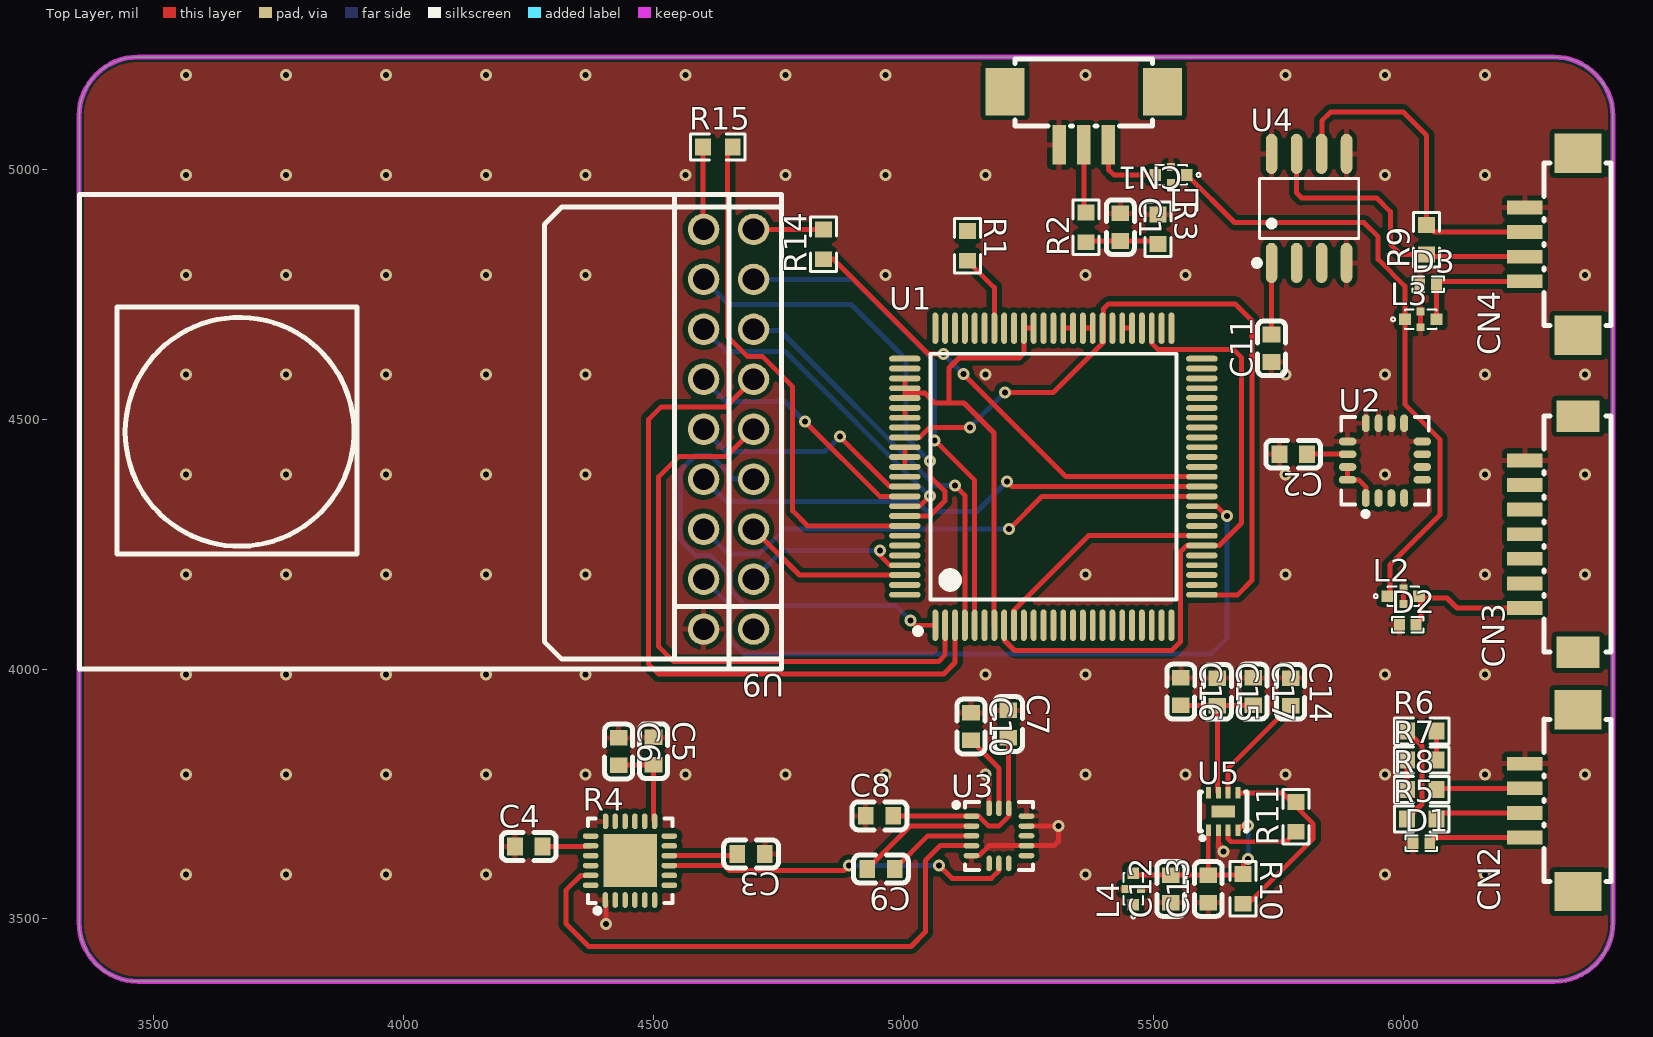
[diagram p0: Top Layer view]
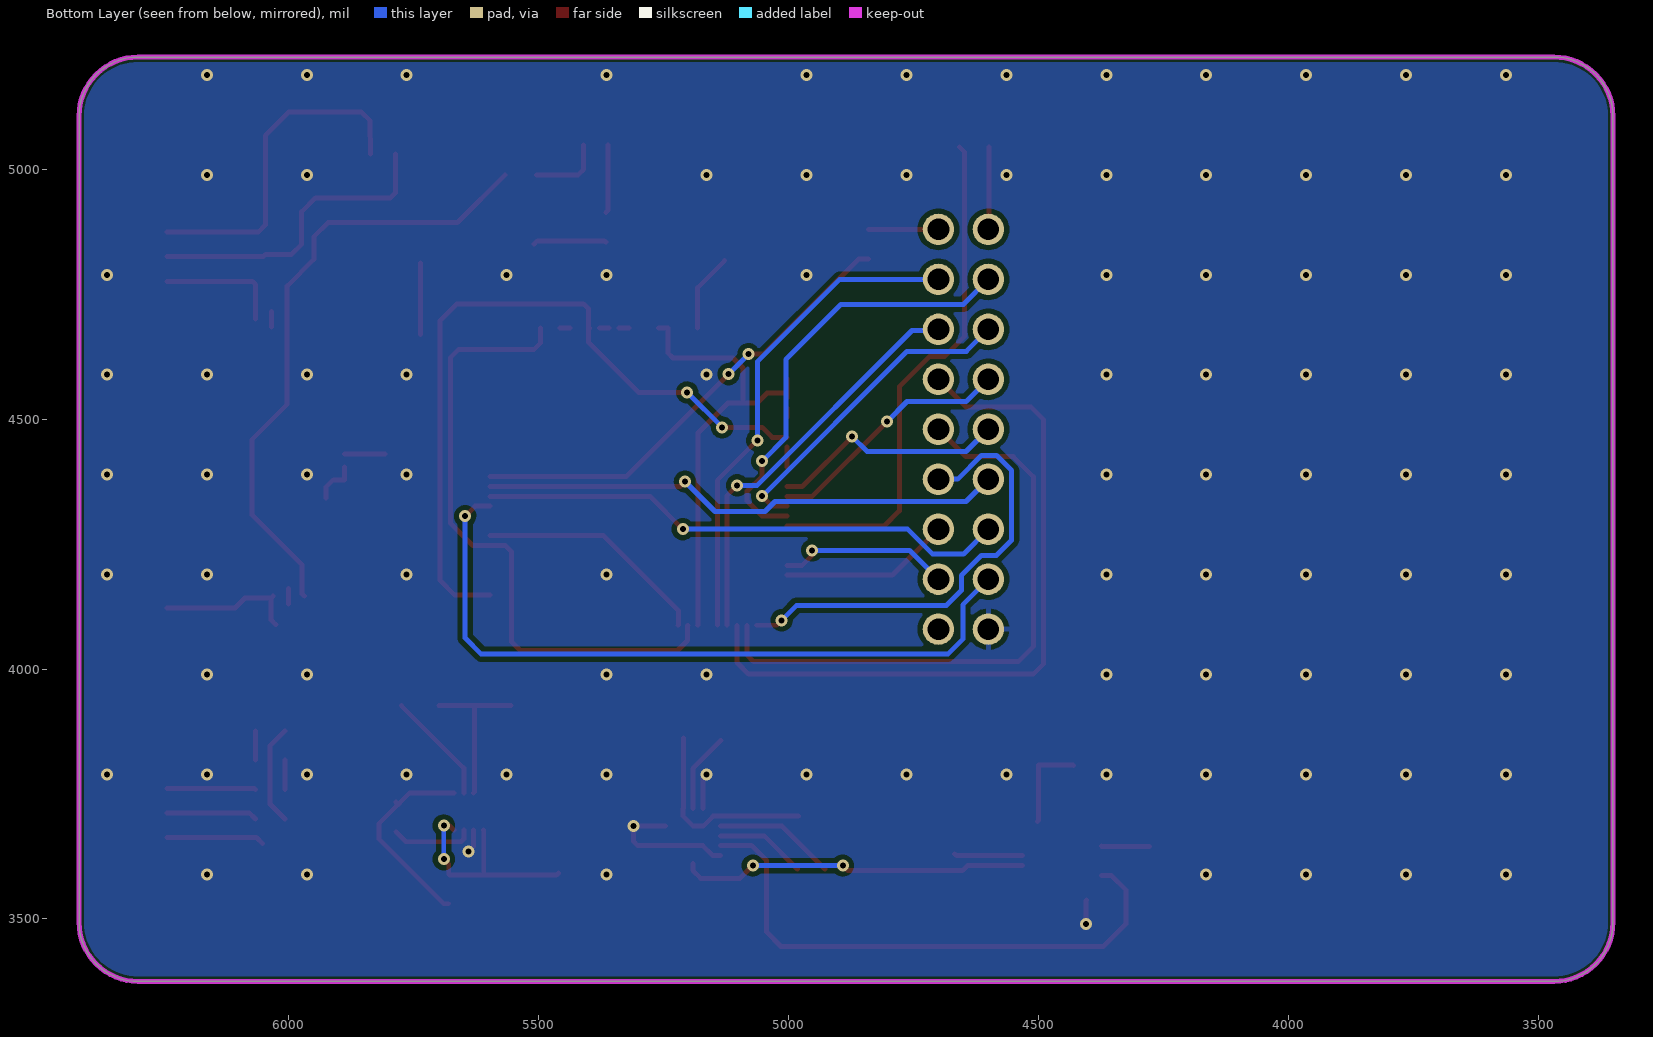
[diagram p1: Bottom Layer view, seen from below]
# Altium PCB MISC50255.pcbdoc
Units mil, origin at the board's own origin, x right, y up, seen from the top; angles counter-clockwise.
Board outline 3070 x 1850 mil, 2 copper layers (Top Layer, Bottom Layer), stack 62.206 mil thick; 47 components, 113 nets, 298 pads, 113 vias.

## Layer stack, top to bottom
Top Solder Mask Layer: solder mask 0.394, Dk 3.3
Top Layer: signal copper 1.379
Dielectric1: surface 59.449, FR4, Dk 4.5
Bottom Layer: signal copper 1.378
Bottom Solder Mask Layer: solder mask 0.394, Dk 3.3

## Board outline
3468.11,5225 ccw(c3468.11,5106.89) 3350,5106.89 3350,3493.11 ccw(c3468.11,3493.11) 3468.11,3375 6301.89,3375 ccw(c6301.89,3493.11) 6420,3493.11 6420,5106.89 ccw(c6301.89,5106.89) 6301.89,5225

## Design rules (kind name [scope] priority, off if disabled: settings)
BoardOutlineClearance copperThickness2oz_1 [All] p2 off: genericclearance=7.99 ignorepadtopadclearanceinfootprint=FALSE except(0: Arc-SplitContinuation Track-SplitContinuation SMDPad-SplitContinuation THPad-SplitContinuation Via-SplitContinuation Fill-SplitContinuation Region-SplitContinuation Poly-SplitContinuation Text-SplitContinuation Hole-SplitContinuation; 5.98: Arc-CutoutEdge Track-CutoutEdge SMDPad-CutoutEdge THPad-CutoutEdge Via-CutoutEdge Text-CutoutEdge; 6.9: Hole-OutlineEdge Hole-CutoutEdge; 10: Poly-OutlineEdge Poly-CutoutEdge; 11.81: Arc-OutlineEdge Track-OutlineEdge SMDPad-OutlineEdge THPad-OutlineEdge Via-OutlineEdge Fill-OutlineEdge Region-OutlineEdge Text-OutlineEdge Fill-CutoutEdge Region-CutoutEdge)
BoardOutlineClearance Plane_innerPlane_1 [All] p4 off: genericclearance=4.02 ignorepadtopadclearanceinfootprint=FALSE except(0: Arc-SplitContinuation Track-SplitContinuation SMDPad-SplitContinuation THPad-SplitContinuation Via-SplitContinuation Fill-SplitContinuation Region-SplitContinuation Poly-SplitContinuation Text-SplitContinuation Hole-SplitContinuation; 5.98: Arc-CutoutEdge Track-CutoutEdge SMDPad-CutoutEdge THPad-CutoutEdge Via-CutoutEdge Text-CutoutEdge; 6.9: Hole-OutlineEdge Hole-CutoutEdge; 10: Poly-OutlineEdge Poly-CutoutEdge; 11.81: Arc-OutlineEdge Track-OutlineEdge SMDPad-OutlineEdge THPad-OutlineEdge Via-OutlineEdge Fill-OutlineEdge Region-OutlineEdge Text-OutlineEdge Fill-CutoutEdge Region-CutoutEdge)
BoardOutlineClearance Copper_copperRegion_1 [All] p6 off: genericclearance=4.02 ignorepadtopadclearanceinfootprint=FALSE except(0: Arc-SplitContinuation Track-SplitContinuation SMDPad-SplitContinuation THPad-SplitContinuation Via-SplitContinuation Fill-SplitContinuation Region-SplitContinuation Poly-SplitContinuation Text-SplitContinuation Hole-SplitContinuation; 5.98: Arc-CutoutEdge Track-CutoutEdge SMDPad-CutoutEdge THPad-CutoutEdge Via-CutoutEdge Text-CutoutEdge; 6.9: Hole-OutlineEdge Hole-CutoutEdge; 10: Poly-OutlineEdge Poly-CutoutEdge; 11.81: Arc-OutlineEdge Track-OutlineEdge SMDPad-OutlineEdge THPad-OutlineEdge Via-OutlineEdge Fill-OutlineEdge Region-OutlineEdge Text-OutlineEdge Fill-CutoutEdge Region-CutoutEdge)
BoardOutlineClearance copperThickness1oz_1 [All] p8: genericclearance=4.02 ignorepadtopadclearanceinfootprint=FALSE except(0: Arc-SplitContinuation Track-SplitContinuation SMDPad-SplitContinuation THPad-SplitContinuation Via-SplitContinuation Fill-SplitContinuation Region-SplitContinuation Poly-SplitContinuation Text-SplitContinuation Hole-SplitContinuation; 5.98: Arc-CutoutEdge Track-CutoutEdge SMDPad-CutoutEdge THPad-CutoutEdge Via-CutoutEdge Text-CutoutEdge; 6.9: Hole-OutlineEdge Hole-CutoutEdge; 10: Poly-OutlineEdge Poly-CutoutEdge; 11.81: Arc-OutlineEdge Track-OutlineEdge SMDPad-OutlineEdge THPad-OutlineEdge Via-OutlineEdge Fill-OutlineEdge Region-OutlineEdge Text-OutlineEdge Fill-CutoutEdge Region-CutoutEdge)
Clearance copperThickness2oz [All] p1 off: gap=7.99 ignorepadtopadclearanceinfootprint=FALSE except(5.98: SMDPad-Track SMDPad-SMDPad THPad-Track SMDPad-THPad THPad-THPad Track-Via SMDPad-Via THPad-Via Via-Via Fill-SMDPad Region-SMDPad Fill-THPad Region-THPad Fill-Via Region-Via Fill-Fill Fill-Region Region-Region Arc-Track Arc-SMDPad Arc-THPad Arc-Via Fill-Arc Region-Arc Arc-Arc Text-Track SMDPad-Text Text-THPad Text-Via Fill-Text Region-Text Arc-Text Text-Text; 6.9: Hole-Track Hole-SMDPad Hole-THPad Hole-Via Fill-Hole Region-Hole Hole-Arc Hole-Text; 10: Poly-Track Poly-SMDPad Poly-THPad Poly-Via Poly-Fill Poly-Region Poly-Poly Poly-Arc Poly-Text Poly-Hole; 11.81: Fill-Track Region-Track)
Clearance Plane_innerPlane [All] p3 off: gap=4.02 ignorepadtopadclearanceinfootprint=FALSE except(5.98: SMDPad-Track SMDPad-SMDPad THPad-Track SMDPad-THPad THPad-THPad Track-Via SMDPad-Via THPad-Via Via-Via Fill-SMDPad Region-SMDPad Fill-THPad Region-THPad Fill-Via Region-Via Fill-Fill Fill-Region Region-Region Arc-Track Arc-SMDPad Arc-THPad Arc-Via Fill-Arc Region-Arc Arc-Arc Text-Track SMDPad-Text Text-THPad Text-Via Fill-Text Region-Text Arc-Text Text-Text; 6.9: Hole-Track Hole-SMDPad Hole-THPad Hole-Via Fill-Hole Region-Hole Hole-Arc Hole-Text; 10: Poly-Track Poly-SMDPad Poly-THPad Poly-Via Poly-Fill Poly-Region Poly-Poly Poly-Arc Poly-Text Poly-Hole; 11.81: Fill-Track Region-Track)
Clearance Copper_copperRegion [All] p5 off: gap=4.02 ignorepadtopadclearanceinfootprint=FALSE except(5.98: SMDPad-Track SMDPad-SMDPad THPad-Track SMDPad-THPad THPad-THPad Track-Via SMDPad-Via THPad-Via Via-Via Fill-SMDPad Region-SMDPad Fill-THPad Region-THPad Fill-Via Region-Via Fill-Fill Fill-Region Region-Region Arc-Track Arc-SMDPad Arc-THPad Arc-Via Fill-Arc Region-Arc Arc-Arc Text-Track SMDPad-Text Text-THPad Text-Via Fill-Text Region-Text Arc-Text Text-Text; 6.9: Hole-Track Hole-SMDPad Hole-THPad Hole-Via Fill-Hole Region-Hole Hole-Arc Hole-Text; 10: Poly-Track Poly-SMDPad Poly-THPad Poly-Via Poly-Fill Poly-Region Poly-Poly Poly-Arc Poly-Text Poly-Hole; 11.81: Fill-Track Region-Track)
Clearance copperThickness1oz [All] p7: gap=4.02 ignorepadtopadclearanceinfootprint=FALSE except(5.98: SMDPad-Track SMDPad-SMDPad THPad-Track SMDPad-THPad THPad-THPad Track-Via SMDPad-Via THPad-Via Via-Via Fill-SMDPad Region-SMDPad Fill-THPad Region-THPad Fill-Via Region-Via Fill-Fill Fill-Region Region-Region Arc-Track Arc-SMDPad Arc-THPad Arc-Via Fill-Arc Region-Arc Arc-Arc Text-Track SMDPad-Text Text-THPad Text-Via Fill-Text Region-Text Arc-Text Text-Text; 6.9: Hole-Track Hole-SMDPad Hole-THPad Hole-Via Fill-Hole Region-Hole Hole-Arc Hole-Text; 10: Poly-Track Poly-SMDPad Poly-THPad Poly-Via Poly-Fill Poly-Region Poly-Poly Poly-Arc Poly-Text Poly-Hole; 11.81: Fill-Track Region-Track)
DiffPairsRouting differentialPair [All] p1: maxlimit=6 minlimit=6 mostfreqgap=6 toplayer_minwidth=5 toplayer_prefwidth=10 toplayer_maxwidth=100 toplayer_mingap=6 toplayer_prefgap=6 toplayer_maxgap=6 bottomlayer_minwidth=5 bottomlayer_prefwidth=10 bottomlayer_maxwidth=100 bottomlayer_mingap=6 bottomlayer_prefgap=6 bottomlayer_maxgap=6 maxuncoupledlength=10
HoleToHoleClearance otherClearance [All] p1: gap=11.81 allowstackedmicrovias=TRUE
Length netLength [All] p1: minlimit=0 maxlimit=0
PasteMaskExpansion pasteMaskExpansion [All] p1: expansion=0
PlaneConnect innerPlane [All] p1: planeconnectstyle=Relief reliefexpansion=20 reliefentries=4 reliefconductorwidth=10 reliefairgap=10
PolygonConnect copperRegion [All] p1: connectstyle=Relief reliefconductorwidth=10 reliefentries=4 polygonreliefangle="90 Angle" airgapwidth=10 via.connectstyle=Relief via.reliefconductorwidth=10 via.reliefentries=4 via.polygonreliefangle="90 Angle" via.airgapwidth=10
RoutingVias viaSize [All] p1: holewidth=12.01 width=24.02 viastyle="Through Hole" minholewidth=11.81 minwidth=19.68 maxholewidth=248.03 maxwidth=393.7
SolderMaskExpansion solderMaskExpansion [IsVia] p1: expansion=-1000 istentingtop=TRUE
SolderMaskExpansion solderMaskExpansion [All] p2: expansion=2 istentingtop=FALSE
Width copperThickness2oz_2 [All] p1 off: maxlimit=100 minlimit=8 preferedwidth=10
Width copperThickness1oz_2 [All] p2: maxlimit=100 minlimit=5 preferedwidth=10

## Components (designator, comment, footprint, x,y, rotation, side; value= is the part's Value field where it differs from the comment)
C1 "100nF" C0603 5433.99,4884.53 r270 top
C2 "10nF" C0603 5780,4430 r180 top
C3 "2U2" C0603 4695,3630 r180 top
C4 "2U2" C0603 4250,3645 r0 top
C5 "2U2" C0603 4499.92,3835.89 r270 top
C6 "0U1" C0603 4430,3835 r270 top
C7 "10UF" C0603 5210,3890 r270 top
C8 "10UF" C0603 4952.03,3706.27 r0 top
C9 "10UF" C0603 4955,3600 r180 top
C10 "10UF" C0603 5135,3885 r270 top
C11 "100nF" C0603 5736.72,4642.03 r90 top
C12 "100nF" C0603 5535,3560 r90 top
C13 "100nF" C0603 5610,3560 r90 top
C14 "100nF" C0603 5774.86,3954.38 r270 top
C15 "100nF" C0603 5628.17,3954.38 r270 top
C16 "100nF" C0603 5555,3955 r270 top
C17 "100nF" C0603 5700,3955 r270 top
CN1 "DF13C-3P-1.25V(51)" CONN-SMD_3P-P1.25_DF13C-3P-1.25V 5360.82,5102.4 r180 top
CN2 "DF13C-4P-1.25V(51)" CONN-SMD_4P-P1.25_DF13C-4P-1.25V 6296.86,3736.86 r90 top
CN3 "DF13C-7P-1.25V(51)" CONN-SMD_7P-P1.25_DF13C-7P-1.25V 6296.86,4270 r90 top
CN4 "DF13C-4P-1.25V(51)" CONN-SMD_4P-P1.25_DF13C-4P-1.25V 6296.86,4850 r90 top
D1 "PESD0402-05ST-ES" DFN1006-2L-BI 6036.51,3651.42 r0 top
D2 "PESD0402-05ST-ES" DFN1006-2L-BI 6009.24,4088.91 r0 top
D3 "PESD0402-05ST-ES" DFN1006-2L-BI 6050,4770 r0 top
L1 "KNH16C104DA5TS" FILTER-SMD_3P-L1.6-W0.8_YFF18PCXXXXXXX 5535.53,4989.03 r180 top
L2 "KNH16C104DA5TS" FILTER-SMD_3P-L1.6-W0.8_YFF18PCXXXXXXX 6000.37,4145.95 r0 top
L3 "KNH16C104DA5TS" FILTER-SMD_3P-L1.6-W0.8_YFF18PCXXXXXXX 6035,4700 r0 top
L4 "KNH16C104DA5TS" FILTER-SMD_3P-L1.6-W0.8_YFF18PCXXXXXXX 5460,3560 r90 top
R1 "10K" R0603 5127.87,4847.02 r270 top
R2 "10K" R0603 5365.53,4884.03 r90 top
R3 "10K" R0603 5508.97,4880.31 r270 top
R4 "MPU-6000" QFN-24_L4.0-W4.0-P0.50-BL-EP2.7 4452.65,3616.63 r0 top
R5 "120R" R0603 6037.28,3700 r0 top
R6 "120R" R0603 6037.28,3876.42 r0 top
R7 "120R" R0603 6037.28,3817.61 r0 top
R8 "120R" R0603 6037.28,3758.81 r0 top
R9 "120R" R0603 6046.83,4859.48 r90 top
R10 "120R" R0603 5680,3560 r270 top
R11 "10K" R0603 5785.47,3704.08 r90 top
R14 "10K" R0603 4840,4850 r90 top
R15 "10K" R0603 4628.56,5045.17 r0 top
U1 "STM32F427VGT6" LQFP-100_L14.0-W14.0-P0.50-LS16.0-BL 5300,4385 r0 top
U2 "L3GD20" LGA-16_L4.0-W4.0-P0.65-BL 5963.7,4417.23 r0 top
U3 "LSM303D" LGA-16_L3.0-W3.0-P0.50-TL 5191.1,3666.27 r0 top
U4 "MAX3051ESA+T" SOIC-8_L4.9-W3.9-P1.27-LS6.0-BL 5811.72,4922.03 r0 top
U5 "MIC5332-PPYMT-TR" MLF-8_L2.0-W2.0-P0.50-BL-EP 5640,3715 r0 top
U9 "OV2640 Camera Board" SENSORM-TH_L35.7-W3.9-OV2640 4650,4480 r180 top

## Footprints (in the part's own frame and the unit in brackets; to place one, negate y for a bottom-side part, rotate by r counter-clockwise, add the part's x,y. Pads: shape width x height; smd on the part's side, far side on the other; paste and mask are expansions set on the pad)
C0603 [mm]
  rect 0.8x0.9 smd: 1(-0.7,0) 2(0.7,0)
  silkscreen extent -1.39,-0.71 1.39,0.71
CONN-SMD_3P-P1.25_DF13C-3P-1.25V [mm]
  rect 0.7x2 smd: 1(-1.25,1.35) 2(0,1.35) 3(1.25,1.35)
  rect 2x2.4 smd: 4(4,-1.35) 5(-4,-1.35)
  silkscreen extent -3.5,-3.02 3.5,0.38
CONN-SMD_4P-P1.25_DF13C-4P-1.25V [mm]
  rect 0.7x1.8 smd: 1(-1.875,1.35) 2(-0.625,1.35) 3(0.625,1.35) 4(1.875,1.35)
  rect 2x2.4 smd: 5(4.625,-1.35) 6(-4.625,-1.35)
  silkscreen extent -4.13,-3.02 4.14,0.38
CONN-SMD_7P-P1.25_DF13C-7P-1.25V [mm]
  rect 0.7x1.8 smd paste+0 mask+0.05: 1(-3.75,1.35) 2(-2.5,1.35) 3(-1.25,1.35) 4(0,1.35) 5(1.25,1.35) 6(2.5,1.35) 7(3.75,1.35)
  rect 1.6x2.2 smd paste+0 mask+0.05: 8(6,-1.35) 9(-6,-1.35)
  silkscreen extent -6,-3.02 6,0.38
DFN1006-2L-BI [mm]
  rect 0.55x0.6 smd: 1(-0.425,0) 2(0.425,0)
  silkscreen extent -0.8,-0.4 0.8,0.4
FILTER-SMD_3P-L1.6-W0.8_YFF18PCXXXXXXX [mm]
  rect 0.6x0.6 smd: 1(-0.8,0) 3(0.8,0)
  rect 0.4x0.4 smd: 2(0,0.4) 2(0,-0.4)
  silkscreen extent -1.5,-0.5 0.8,0.5
LGA-16_L3.0-W3.0-P0.50-TL [mm]
  oval 0.8x0.28 smd: 1(-1.4,1) 2(-1.4,0.5) 3(-1.4,0) 4(-1.4,-0.5) 5(-1.4,-1) 9(1.4,-1) 10(1.4,-0.5) 11(1.4,0) 12(1.4,0.5) 13(1.4,1)
  oval 0.28x0.8 smd: 6(-0.5,-1.4) 7(0,-1.4) 8(0.5,-1.4) 14(0.5,1.4) 15(0,1.4) 16(-0.5,1.4)
  silkscreen extent -2.3,-1.72 1.73,1.73
LGA-16_L4.0-W4.0-P0.65-BL [mm]
  oval 0.4x0.9 smd: 1(-0.975,-1.9) 2(-0.325,-1.9) 3(0.325,-1.9) 4(0.975,-1.9) 9(0.975,1.9) 10(0.325,1.9) 11(-0.325,1.9) 12(-0.975,1.9)
  oval 0.9x0.4 smd: 5(1.9,-0.975) 6(1.9,-0.325) 7(1.9,0.325) 8(1.9,0.975) 13(-1.9,0.975) 14(-1.9,0.325) 15(-1.9,-0.325) 16(-1.9,-0.975)
  silkscreen extent -2.22,-2.84 2.22,2.22
LQFP-100_L14.0-W14.0-P0.50-LS16.0-BL [mm]
  oval 0.3x1.6 smd: 1(-6,-7.55) 2(-5.5,-7.55) 3(-5,-7.55) 4(-4.5,-7.55) 5(-4,-7.55) 6(-3.5,-7.55) 7(-3,-7.55) 8(-2.5,-7.55) 9(-2,-7.55) 10(-1.5,-7.55) 11(-1,-7.55) 12(-0.5,-7.55) 13(0,-7.55) 14(0.5,-7.55) 15(1,-7.55) 16(1.5,-7.55) 17(2,-7.55) 18(2.5,-7.55) 19(3,-7.55) 20(3.5,-7.55) 21(4,-7.55) 22(4.5,-7.55) 23(5,-7.55) 24(5.5,-7.55) 25(6,-7.55) 51(6,7.55) 52(5.5,7.55) 53(5,7.55) 54(4.5,7.55) 55(4,7.55) 56(3.5,7.55) 57(3,7.55) 58(2.5,7.55) 59(2,7.55) 60(1.5,7.55) 61(1,7.55) 62(0.5,7.55) 63(0,7.55) 64(-0.5,7.55) 65(-1,7.55) 66(-1.5,7.55) 67(-2,7.55) 68(-2.5,7.55) 69(-3,7.55) 70(-3.5,7.55) 71(-4,7.55) 72(-4.5,7.55) 73(-5,7.55) 74(-5.5,7.55) 75(-6,7.55)
  oval 1.6x0.3 smd: 26(7.55,-6) 27(7.55,-5.5) 28(7.55,-5) 29(7.55,-4.5) 30(7.55,-4) 31(7.55,-3.5) 32(7.55,-3) 33(7.55,-2.5) 34(7.55,-2) 35(7.55,-1.5) 36(7.55,-1) 37(7.55,-0.5) 38(7.55,0) 39(7.55,0.5) 40(7.55,1) 41(7.55,1.5) 42(7.55,2) 43(7.55,2.5) 44(7.55,3) 45(7.55,3.5) 46(7.55,4) 47(7.55,4.5) 48(7.55,5) 49(7.55,5.5) 50(7.55,6) 76(-7.55,6) 77(-7.55,5.5) 78(-7.55,5) 79(-7.55,4.5) 80(-7.55,4) 81(-7.55,3.5) 82(-7.55,3) 83(-7.55,2.5) 84(-7.55,2) 85(-7.55,1.5) 86(-7.55,1) 87(-7.55,0.5) 88(-7.55,0) 89(-7.55,-0.5) 90(-7.55,-1) 91(-7.55,-1.5) 92(-7.55,-2) 93(-7.55,-2.5) 94(-7.55,-3) 95(-7.55,-3.5) 96(-7.55,-4) 97(-7.55,-4.5) 98(-7.55,-5) 99(-7.55,-5.5) 100(-7.55,-6)
  silkscreen extent -7.03,-8 6.25,6.25
MLF-8_L2.0-W2.0-P0.50-BL-EP [mm]
  rect 0.25x0.6 smd: 1(-0.75,-0.95) 2(-0.25,-0.95) 3(0.25,-0.95) 4(0.75,-0.95) 5(0.75,0.95) 6(0.25,0.95) 7(-0.25,0.95) 8(-0.75,0.95)
  rect 1.2x0.6 smd: 9(0,0)
  silkscreen extent -1.2,-1.45 1.2,1
QFN-24_L4.0-W4.0-P0.50-BL-EP2.7 [mm]
  oval 0.28x0.8 smd paste-100 mask+0.05: 1(-1.25,-2) 2(-0.75,-2) 3(-0.25,-2) 4(0.25,-2) 5(0.75,-2) 6(1.25,-2) 13(1.25,2) 14(0.75,2) 15(0.25,2) 16(-0.25,2) 17(-0.75,2) 18(-1.242,2)
  oval 0.8x0.28 smd paste-100 mask+0.05: 7(2,-1.25) 8(2,-0.75) 9(2,-0.25) 10(2,0.25) 11(2,0.75) 12(2,1.25) 19(-2,1.25) 20(-2,0.75) 21(-2,0.25) 22(-2,-0.25) 23(-2,-0.75) 24(-2,-1.25)
  rect 2.7x2.7 smd paste-100 mask+0.05: 25(0.012,0)
  silkscreen extent -2.14,-2.79 2.16,2.15
R0603 [mil]
  rect 31.75x34.02 smd paste-3937.01 mask+2: 1(-29.66,0) 2(29.66,0)
  silkscreen extent -55,-26 55,26
SENSORM-TH_L35.7-W3.9-OV2640 [mm]
  round 1.6 hole 1.1 paste+0 mask+0.05: 1(-1.27,10.16) 2(-1.27,7.62) 3(-1.27,5.08) 4(-1.27,2.54) 5(-1.27,0) 6(-1.27,-2.54) 7(-1.27,-5.08) 8(-1.27,-7.62) 9(-1.27,-10.16) 10(1.27,-10.16) 11(1.27,-7.62) 12(1.27,-5.08) 13(1.27,-2.54) 14(1.27,0) 15(1.27,2.54) 16(1.27,5.08) 17(1.27,7.62) 18(1.27,10.16)
  silkscreen extent -2.7,-11.94 32.99,12.19
SOIC-8_L4.9-W3.9-P1.27-LS6.0-BL [mm]
  oval 0.588x2.045 smd: 1(-1.905,-2.772) 2(-0.635,-2.772) 3(0.635,-2.772) 4(1.905,-2.772) 5(1.905,2.772) 6(0.635,2.772) 7(-0.635,2.772) 8(-1.905,2.772)
  silkscreen extent -2.8,-2.92 2.53,1.52

## Via types
v1: diameter 24.02, hole 12, Top Layer to Bottom Layer, 113 vias

## Nets (pads, with @x,y where several pads share a name; then routed paths per layer and width w, separated by ;. In a path a pad name is that pad's centre, name@x,y a point inside that pad or via, vN(x,y) a via of type N, cw(c..) or ccw(c..) an arc to the next point about the centre after c; other vN are vias at no path point)
$1N877: R1.2 U1.69 | length 157.5
  Top Layer w10: R1.2 5181.89,4763.34 U1.69
$1N1241: CN1.1 L1.3 | length 147.8
  Top Layer w10: CN1.1 5410.03,4999.97 5420.97,4989.03 L1.3
$1N1807: C2.1 U2.14 | length 81.3
  Top Layer w10: C2.1 U2.14
$1N2279: C3.2 R4.10 | length 137.5
  Top Layer w10: R4.10 4663.91,3626.47 C3.2
$1N2414: C4.2 R4.20 | length 96.8
  Top Layer w10: C4.2 4372.75,3645 R4.20
$1N3306: C9.1 U3.3 | length 180.9
  Top Layer w10: C9.1 5048.84,3666.28 U3.3
$1N3316: C9.2 U3.2 | length 244.1
  Top Layer w10: C9.2 5013.4,3685.96 U3.2
$1N3418: C10.2 U3.15 | length 159.3
  Top Layer w10: C10.2 5191.1,3801.34 U3.15
$1N3634: CN2.1 D1.2 | length 195.3
  Top Layer w10: D1.2 6064.85,3663.04 CN2.1
$1N3639: CN2.2 R5.2 | length 181.8
  Top Layer w10: R5.2 6079.19,3712.25 CN2.2
$1N3808: CN2.3 R8.2 | length 177.9
  Top Layer w10: R8.2 6069.59,3761.46 CN2.3
$1N4095: CN3.1 D2.2 L2.3 | length 279
  Top Layer w10: D2.2 6035.47,4098.4 L2.3@6035.47,4142.36 ; L2.3 L2.3@6035.47,4142.36 ; CN3.1 6107.64,4122.36 6087.64,4142.36 L2.3@6035.47,4142.36
$1N4583: CN4.1 D3.2 L3.3 | length 249.3
  Top Layer w10: L3.3@6066.73,4700.23 D3.2 6072.9,4776.18 CN4.1
$1N6097: C12.2 C13.2 L4.3 R10.1 U5.1 U5.4 | length 438.8
  Top Layer w9.84: C13.2 5610,3677.13 U5.1 ; U5.4 5679.06,3687.13 v1(5690,3687.13) ; R10.1 5680,3609.66 v1(5690,3619.66)
  Top Layer w10: L4.3 5463.94,3587.56 C12.2 C13.2 5677.9,3587.56 R10.1
  Bottom Layer w9.84: v1(5690,3619.66) v1(5690,3687.13)
$1N6348: C14.2 U5.6 | length 226.2
  Top Layer w9.84: U5.6 5649.84,3801.8 C14.2
$1N10490: R14.2 U9.9 | length 140.1
  Top Layer w10: U9.9 4700.34,4879.66 R14.2
$1N10540: R15.1 U9.10 | length 165.6
  Top Layer w10: R15.1 4598.9,4881.1 U9.10
(RPUCS/5.1C: U1.17
ACCELDRDY/1.1B: U3.11
ACCELHAGCS/1.3B: U3.8
ALARM/7.10: U1.77
BAROCS/5.40: U1.88
BATT_CURRENT_SENS//11.2C: U1.26 U1.58 U1.84 | length 1492.4
  Top Layer w10: U1.84 5032.76,4463.74 5052.76,4483.74 v1(5132.76,4483.74) ; v1(5202.76,4553.74) 5299.93,4553.74 5399.93,4653.74 U1.58@5399.93,4680.74 ; U1.58 U1.58@5399.93,4680.74 ; U1.26 5668.78,4148.78 5697.24,4177.24 5697.24,4697.76 5664.26,4730.74 5409.93,4730.74 5399.93,4720.74 U1.58@5399.93,4680.74
  Bottom Layer w10: v1(5132.76,4483.74) v1(5202.76,4553.74)
BATT_VOLTAGE_SENS/11.2C: U1.25
CAN1-X/4.4C: U1.81 U1.82 | length 19.7
  Top Layer w10: U1.82 U1.81
CAN1_RX/1.3B: U4.3
CAN1TX/1.3B: U4.2
CAN2RX/2.4C: U1.51
CANH/12.3C: CN4.2 R9.1 U4.7 | length 625.9
  Top Layer w10: U4.7 5786.72,4953.28 5796.72,4943.28 5946.72,4943.28 5974.43,4915.57 5974.43,4850.57 5995.18,4829.82 R9.1 6051.27,4825.39 CN4.2
CANL/12.3C: CN4.3 R9.2 U4.6 | length 684.4
  Top Layer w10: U4.6 5837.14,5097.14 5855,5115 6000,5115 6046.83,5068.17 R9.2 6061.38,4874.6 CN4.3
CBUSUALID/11.6C: U1.15
CU003U3SENS0RS/12.6A: U5.8
D2: U1.92 U9.11 | length 879.6
  Top Layer w10: U1.92 5052.76,4306.26 5082.76,4336.26 5082.76,4356.26 5052.76,4386.26 v1(5052.76,4416.26)
  Bottom Layer w10: U9.11 4650,4730 4895,4730 5005,4620 5005,4464.02 v1(5052.76,4416.26)
D3: U1.5 U9.8 | length 991.4
  Top Layer w10: v1(5062.52,4457.76) 5142.52,4377.76 U1.5
  Bottom Layer w10: U9.8 4897.82,4780 5062.52,4615.3 v1(5062.52,4457.76)
D4: U1.91 U9.12 | length 649.4
  Top Layer w10: U1.91 5032.76,4325.94 v1(5052.76,4345.94)
  Bottom Layer w10: U9.12 4644.06,4635.94 4762.76,4635.94 v1(5052.76,4345.94)
D5: U1.4 U9.7 | length 820.4
  Top Layer w10: v1(5102.83,4367.76) 5122.83,4347.76 U1.4
  Bottom Layer w10: U9.7 4702.24,4677.76 4752.83,4677.76 5062.83,4367.76 v1(5102.83,4367.76)
D6: U1.90 U9.13 | length 499.8
  Top Layer w10: v1(4802.76,4495.63) 4952.76,4345.63 U1.90
  Bottom Layer w10: U9.13 4644.37,4535.63 4762.76,4535.63 v1(4802.76,4495.63)
D7: U1.3 U9.6 | length 1438.8
  Top Layer w10: U9.6 4645,4525 4515,4525 4490,4500 4490,4010 4510,3990 5080,3990 5103.15,4013.15 U1.3
D8: U1.89 U9.14 | length 475.1
  Top Layer w10: v1(4872.76,4465.32) 4972.76,4365.32 U1.89
  Bottom Layer w10: U9.14 4644.68,4435.32 4842.76,4435.32 v1(4872.76,4465.32)
D9: U1.2 U9.5 | length 1220.1
  Top Layer w10: U9.5 4645,4425 4550,4425 4510,4385 4510,4045 4540,4015 5070,4015 5083.46,4028.46 U1.2
FHU-5MCLK/3.5C: U1.76
FHU-12C1SOAV4.10: U1.96
FHU-CHSV9.1A: U1.61 U1.62 | length 19.7
  Top Layer w10: U1.62 U1.61
FHU-RLSET/7.1B: R11.1 U5.3 | length 163.8
  Top Layer w9.84: U5.3 5649.84,3660.05 5655.47,3654.42 5765.47,3654.42 R11.1
FHU-UDD3U3/7.38: C15.2 C16.2 C17.2 U5.7 | length 320.8
  Top Layer w9.84: C15.2 5628.17,3754.39 U5.7
  Top Layer w10: C16.2 5555.62,3926.82 C15.2 5699.38,3926.82 C17.2
FHU-USART2CTS/2.18: U1.85 U1.86 U1.87 | length 39.4
  Top Layer w10: U1.87 U1.86 U1.85
FHU-USART3_CTS/2.1A: U1.59 U1.60 | length 19.7
  Top Layer w10: U1.60 U1.59
FHU-USART3TX/2.1A: U1.55 U1.56 | length 19.7
  Top Layer w10: U1.56 U1.55
FHUAUKADC1/4.48: U1.18
FHUAUKADC2/4.4A: U1.33
FMU-12C1SCL/4.10: U1.95
FMU-12C2_SCL/3.4A: U1.47
FMU-12C2_SDA/3.4A: U1.48
FMU-I2C1_SCL/1.1C: R5.1 R6.1 | length 201.3
  Top Layer w10: R5.1 6037.62,3730 6037.62,3846.42 R6.1
FMU-I2C1_SDA/1.1C: R7.1 R8.1 | length 58.8
  Top Layer w10: R8.1 R7.1
FMU-SHD10/3.5C: U1.72
FMU-UART4_RX/2.1C: U1.24
FMU-UART4_TX/2.1C: U1.23
FMU-UDD_3U3/3.5C: C11.2 U4.1 | length 143.3
  Top Layer w10: C11.2 U4.1
FMU-VDD_3U3/3.50: R6.2 R7.2 | length 58.8
  Top Layer w10: R7.2 R6.2
FRAMCS: U1.57
FRAMMOSI: U1.54
FRAMSCK: U1.52
GND: C1.1 C2.2 C3.1 C4.1 C5.1 C6.1 C7.1 C8.1 C10.1 C11.1 C12.1 C13.1 C14.1 C15.1 C16.1 C17.1 CN1.3 CN2.4 CN3.7 CN4.4 D1.1 D2.1 D3.1 L1.2 L2.2 L3.2 L4.2 R3.1 R4.1 R4.18 U2.8 U2.9 U2.10 U2.11 U2.12 U2.13 U3.5 U3.10 U3.12 U3.13 U3.16 U4.4 U4.5 U4.8 U5.2 U9.18 | length 509.4
  Top Layer w10: R4.1 4405,3536.32 v1(4405,3490) ; U3.5 5151.91,3626.91 5171.59,3646.59 U3.10 5301.59,3646.59 5310,3655 v1(5310,3685.96) U3.12 ; v1(5164.1,3789.1) 5171.42,3781.78 U3.16 ; U5.2 5630.16,3644.84 v1(5640,3635) ; L2.2@6000.37,4130.2 L2.2@6000.37,4161.7 ; L3.2@6035,4684.25 L3.2@6035,4715.75
  other v1: 3564.1,3589.1 3764.1,3589.1 3964.1,3589.1 4164.1,3589.1 5364.1,3589.1 5964.1,3589.1 6164.1,3589.1 3564.1,3789.1 3764.1,3789.1 3964.1,3789.1 4164.1,3789.1 4364.1,3789.1 4564.1,3789.1 4764.1,3789.1 4964.1,3789.1 5364.1,3789.1 5564.1,3789.1 5764.1,3789.1 5964.1,3789.1 6164.1,3789.1 6364.1,3789.1 3564.1,3989.1 3764.1,3989.1 3964.1,3989.1 4164.1,3989.1 4364.1,3989.1 5164.1,3989.1 5364.1,3989.1 5964.1,3989.1 6164.1,3989.1 3564.1,4189.1 3764.1,4189.1 3964.1,4189.1 4164.1,4189.1 4364.1,4189.1 5364.1,4189.1 5764.1,4189.1 6164.1,4189.1 6364.1,4189.1 3564.1,4389.1 3764.1,4389.1 3964.1,4389.1 4164.1,4389.1 4364.1,4389.1 5764.1,4389.1 5964.1,4389.1 6164.1,4389.1 6364.1,4389.1 3564.1,4589.1 3764.1,4589.1 3964.1,4589.1 4164.1,4589.1 4364.1,4589.1 5164.1,4589.1 5764.1,4589.1 5964.1,4589.1 6164.1,4589.1 6364.1,4589.1 3564.1,4789.1 3764.1,4789.1 3964.1,4789.1 4164.1,4789.1 4364.1,4789.1 4964.1,4789.1 5364.1,4789.1 5564.1,4789.1 6364.1,4789.1 3564.1,4989.1 3764.1,4989.1 3964.1,4989.1 4164.1,4989.1 4364.1,4989.1 4564.1,4989.1 4764.1,4989.1 4964.1,4989.1 5164.1,4989.1 5964.1,4989.1 6164.1,4989.1 3564.1,5189.1 3764.1,5189.1 3964.1,5189.1 4164.1,5189.1 4364.1,5189.1 4564.1,5189.1 4764.1,5189.1 4964.1,5189.1 5364.1,5189.1 5764.1,5189.1 5964.1,5189.1 6164.1,5189.1
GPIO_EXT_1/1.3B: CN3.6
GYHODROY/4.1B: U2.6
GYRDCS71.38: U2.5
HREF: U1.36 U9.16 | length 1065.8
  Top Layer w10: v1(5211.61,4280) 5277.24,4345.63 U1.36
  Bottom Layer w10: U9.16 4650,4230 4711.61,4230 4761.61,4280 v1(5211.61,4280)
I0-USART1TX/8.1A: R1.1
MAG_DROY/1.1B: U3.9
NET10: R4.12
OTGFSDH/3.1B: U1.70
OTGFSDP/3.1A: U1.71
PCLK: U1.1 U9.4 | length 916.4
  Top Layer w10: v1(5013.78,4097.76) 5023.78,4087.76 U1.1
  Bottom Layer w10: U9.4 4661.54,4380 4613.78,4427.76 4583.78,4427.76 4553.78,4397.76 4553.78,4257.76 4583.78,4227.76 4613.78,4227.76 4653.78,4187.76 4653.78,4157.76 4683.78,4127.76 4983.78,4127.76 v1(5013.78,4097.76)
PPUCS/1.3A: R4.8
PRESSURE_SENS/1.3A: C1.2 R2.1 R3.2 | length 147.1
  Top Layer w10: R2.1 5368.13,4856.97 C1.2 5502.65,4856.97 R3.2
PRESSURESENS/4.1C: U1.34
PRESSURESENSIN/12.4B: CN1.2 R2.2 | length 137.5
  Top Layer w10: CN1.2 5360.82,4918.4 R2.2
PWDN: R15.2 U1.93 | length 1041
  Top Layer w10: R15.2 4648.22,5035.17 4648.22,4665.17 4688.22,4625.17 4718.22,4625.17 4778.22,4565.17 4778.22,4316.78 4808.43,4286.57 U1.93
RESET: R14.1 U1.38 | length 937.6
  Top Layer w10: R14.1 4860,4820.34 5050,4630.34 v1(5080,4630.34) ; v1(5120,4590.34) 5325.34,4385 U1.38
  Bottom Layer w10: v1(5080,4630.34) v1(5120,4590.34)
S01002/3.1C: U1.7 U1.65 U1.66 U1.78 U1.79 U1.80 | length 937.7
  Top Layer w10: U1.80 5002.76,4552.48 ; U1.78 U1.79 5002.76,4552.48 ; U1.7 5181.18,4088.47 5181.18,4472.48 5121.18,4532.48 5091.18,4532.48 ; U1.65 U1.66 5240.94,4632.24 5231.18,4622.48 5111.18,4622.48 5091.18,4602.48 5091.18,4532.48 ; 5002.76,4552.48 5042.76,4552.48 5062.76,4532.48 5091.18,4532.48
SD10CMD/3.1C: U1.83
SERIALFHUTO10/8.2A: U1.63
SERIALI0TOFHU/8.2A: U1.64
SIO_CLK: U1.97 U9.2 | length 345
  Top Layer w10: v1(4952.76,4237.83) 4952.76,4227.83 4972.76,4207.83 U1.97
  Bottom Layer w10: U9.2 4757.83,4237.83 v1(4952.76,4237.83)
SIO_DAT: U1.35 U9.17 | length 1465
  Top Layer w10: U1.35 5627.24,4325.94 v1(5647.24,4305.94)
  Bottom Layer w10: U9.17 4651.3,4128.7 4651.3,4060 4681.3,4030 5615,4030 5647.24,4062.24 v1(5647.24,4305.94)
SP1INTSCK/3.1A: U2.2
SPAREADC: U1.16
SPI_EXT_MIS0/1.5A: CN3.3
SPI_EXT_MOSI/1.5A: CN3.4
SPI_EXT_SCK/1.5A: CN3.2
SPI_INT_MISO/5.10: U1.8 U1.31 U1.53 | length 1277.8
  Top Layer w10: U1.8 5202.13,4087.2 5202.13,4057.2 5222.13,4037.2 5537.24,4037.2 5554.25,4054.21 5554.25,4234.21 5567.24,4247.2 U1.31 5631.81,4247.2 5676.85,4292.24 5676.85,4623.15 5660.75,4639.25 5509.84,4639.25 5496.85,4652.24 U1.53
SPI_INT_MOSI/5.10: U1.9 U1.32 | length 468.5
  Top Layer w10: U1.9 5220.39,4088.63 5220.39,4116.89 5370.39,4266.89 U1.32
SPI_INT_SCK/5.10: U1.30
SPIEXTNSS/1.5A: CN3.5
SPIINT_HOSI/1.1A: U3.6
SPIINTHISO/1.1A: R4.9 U3.7 | length 699.6
  Top Layer w10: R4.9 4641.39,3606.79 4651.39,3596.79 4881.39,3596.79 v1(4891.39,3606.79) ; v1(5071.39,3606.79) 5097.02,3581.16 5175.75,3581.16 5191.1,3596.51 U3.7
  Bottom Layer w10: v1(4891.39,3606.79) v1(5071.39,3606.79)
SPIINTMOSI/1.1A: R4.24
SPIINTSCK/1.1A: R4.23 U3.4 | length 1126.5
  Top Layer w10: R4.23 4353.9,3587.1 4325,3558.19 4325,3490 4370,3445 5015,3445 5043.9,3473.91 5043.9,3617.1 5073.9,3647.1 5135.47,3647.1 U3.4
SPLINTHOSI/1.1A: U2.3
SPLINTMISO/1.1A: U2.4
U0D3U3_SENSORS/6.30: C5.2 C6.2 R4.13 | length 184.1
  Top Layer w10: C6.2 4430.89,3808.33 C5.2 4499.92,3697.3 R4.13
U005V_PERIPH/2.5C: L1.1 L2.1 L3.1 | length 1247.9
  Top Layer w10: L1.1 5662.39,4893.67 5921.33,4893.67 5950,4865 5950,4820 6003.5,4766.5 L3.1 6003.5,4530 6073.5,4460 6073.5,4308.5 5973.5,4208.5 5973.5,4150.58 L2.1
UBUS/3.1A: U1.68
UDD3U3SENSORSEN/1.5A: R10.2 R11.2 U5.5 | length 406.9
  Top Layer w9.84: U5.5 5757.94,3752.4 R11.2@5780,3730.34 ; R10.2 5690,3530.34 5820,3660.34 5820,3690.34 R11.2@5780,3730.34 ; R11.2 5782.07,3730.34 R11.2@5780,3730.34
UDD_3U3_SENSORS/6.30: C7.2 C8.2 U3.1 U3.14 | length 405.2
  Top Layer w10: C8.2 4980.21,3705.65 U3.1 5150.79,3705.65 5170.79,3685.65 5190.79,3685.65 5210.79,3705.65 U3.14 5210,3722.18 C7.2
UO05U_PERIPH_EN/6.4C: U1.67
UO05UIN/7.1C: L4.1
UOD_3U3_SENSORS/4.30: U2.1 U2.15 U2.16 | length 90.1
  Top Layer w10: U2.15 U2.16 5911.17,4378.83 5925.31,4364.69 U2.1
UOD_5V_SENS/6.6D: U1.29
VCC: U9.1
VSYNC: U1.98 U9.3 | length 340.8
  Top Layer w10: U9.3 4791.85,4188.15 U1.98
XCLK: U1.37 U9.15 | length 1053
  Top Layer w10: v1(5207.24,4375.32) 5217.24,4365.32 U1.37
  Bottom Layer w10: U9.15 4644.68,4335.32 5027.24,4335.32 5047.24,4315.32 5147.24,4315.32 v1(5207.24,4375.32)
pads on no net: CN1.4 CN1.5 CN2.5 CN2.6 CN3.8 CN3.9 CN4.5 CN4.6 R4.2 R4.3 R4.4 R4.5 R4.6 R4.7 R4.11 R4.14 R4.15 R4.16 R4.17 R4.19 R4.21 R4.22 R4.25 U1.6 U1.10 U1.11 U1.12 U1.13 U1.14 U1.19 U1.20 U1.21 U1.22 U1.27 U1.28 U1.39 U1.40 U1.41 U1.42 U1.43 U1.44 U1.45 U1.46 U1.49 U1.50 U1.73 U1.74 U1.75 U1.94 U1.99 U1.100 U2.7 U5.9

## Polygon pours and split planes (outlines as drawn)
GND on Top Layer (solid, remove dead copper, pour order 0): 3000,5615 3000,3000 6720,3000 6720,5615
GND on Bottom Layer (solid, remove dead copper, pour order 2): 3140,5465 3140,3220 6690,3220 6690,5465

## Keep-outs
Board Outline Layer:
  the board outline again, w10